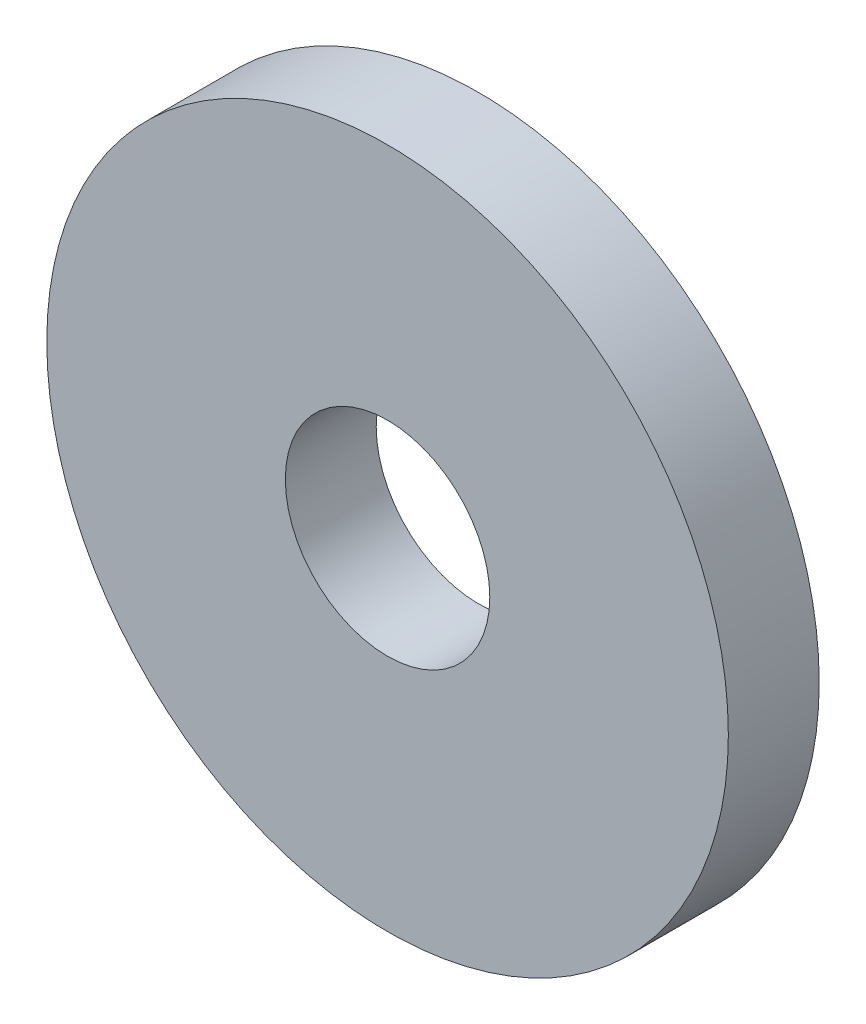
from build123d import *

# Parameters (mm, degrees)
SKETCH_1_R      = 7.5
SKETCH_1_R_2    = 2.25
EXTRUDE_1_DEPTH = 2


with BuildPart() as part:
    # 草图1 → 凸台-拉伸1 (new body)
    with BuildSketch(Plane.XY):
        Circle(SKETCH_1_R)
        Circle(SKETCH_1_R_2, mode=Mode.SUBTRACT)
    extrude(amount=EXTRUDE_1_DEPTH)


solid = part.part
